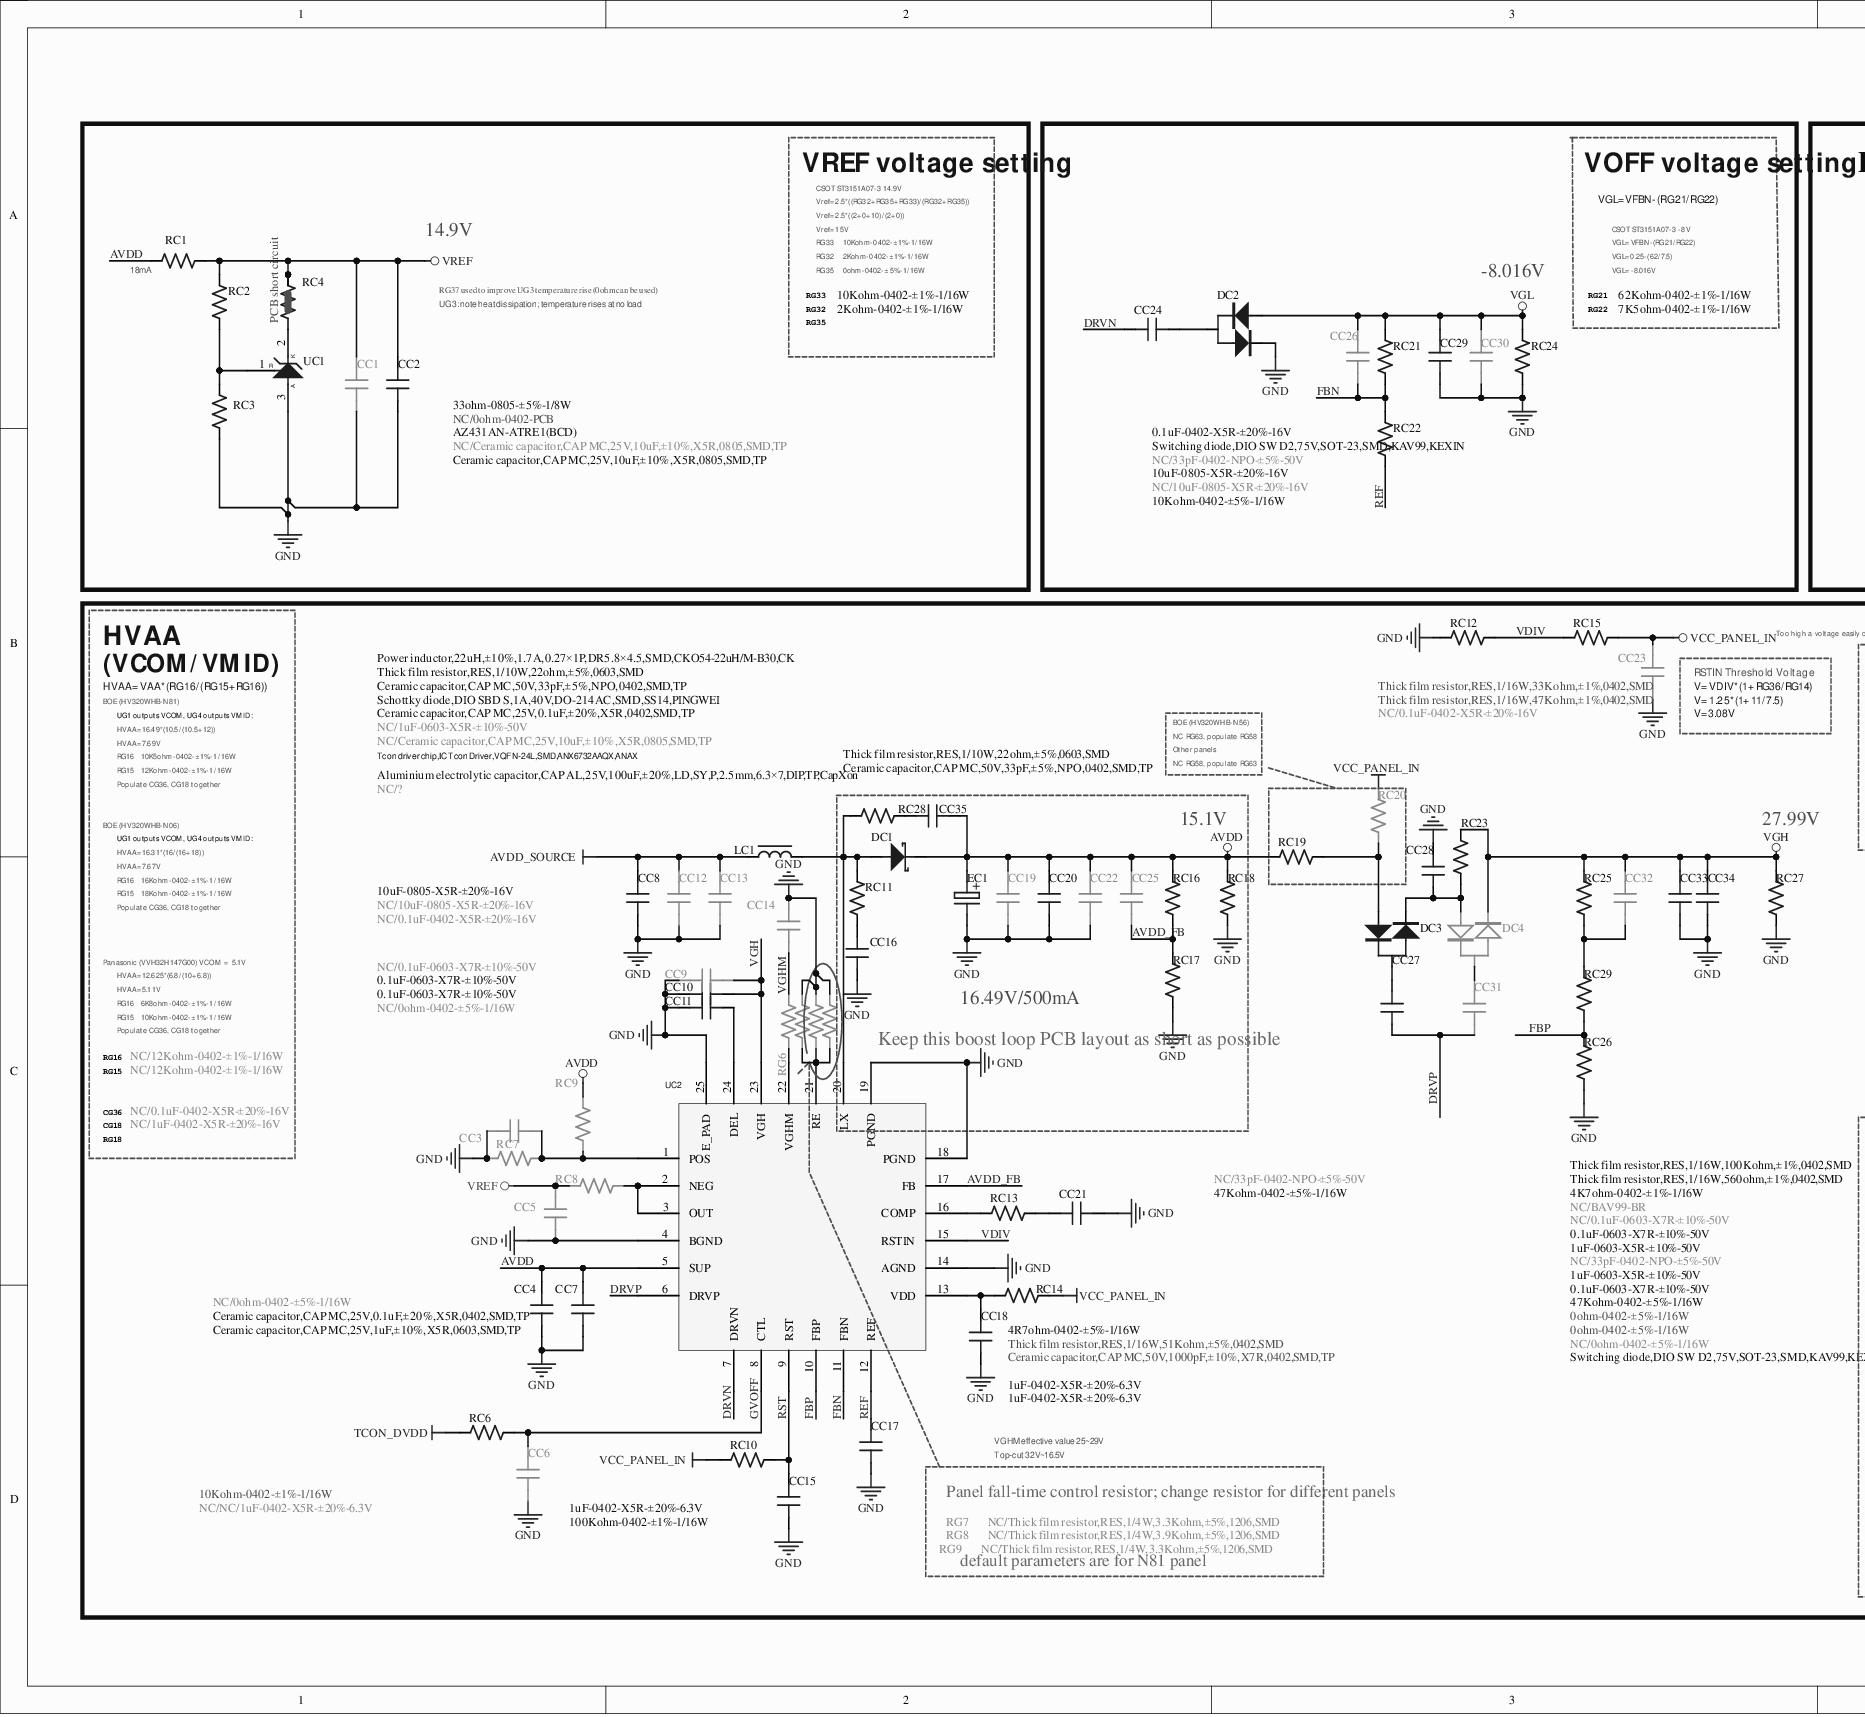
[diagram p0: MISC84395-18.SchDoc, left]
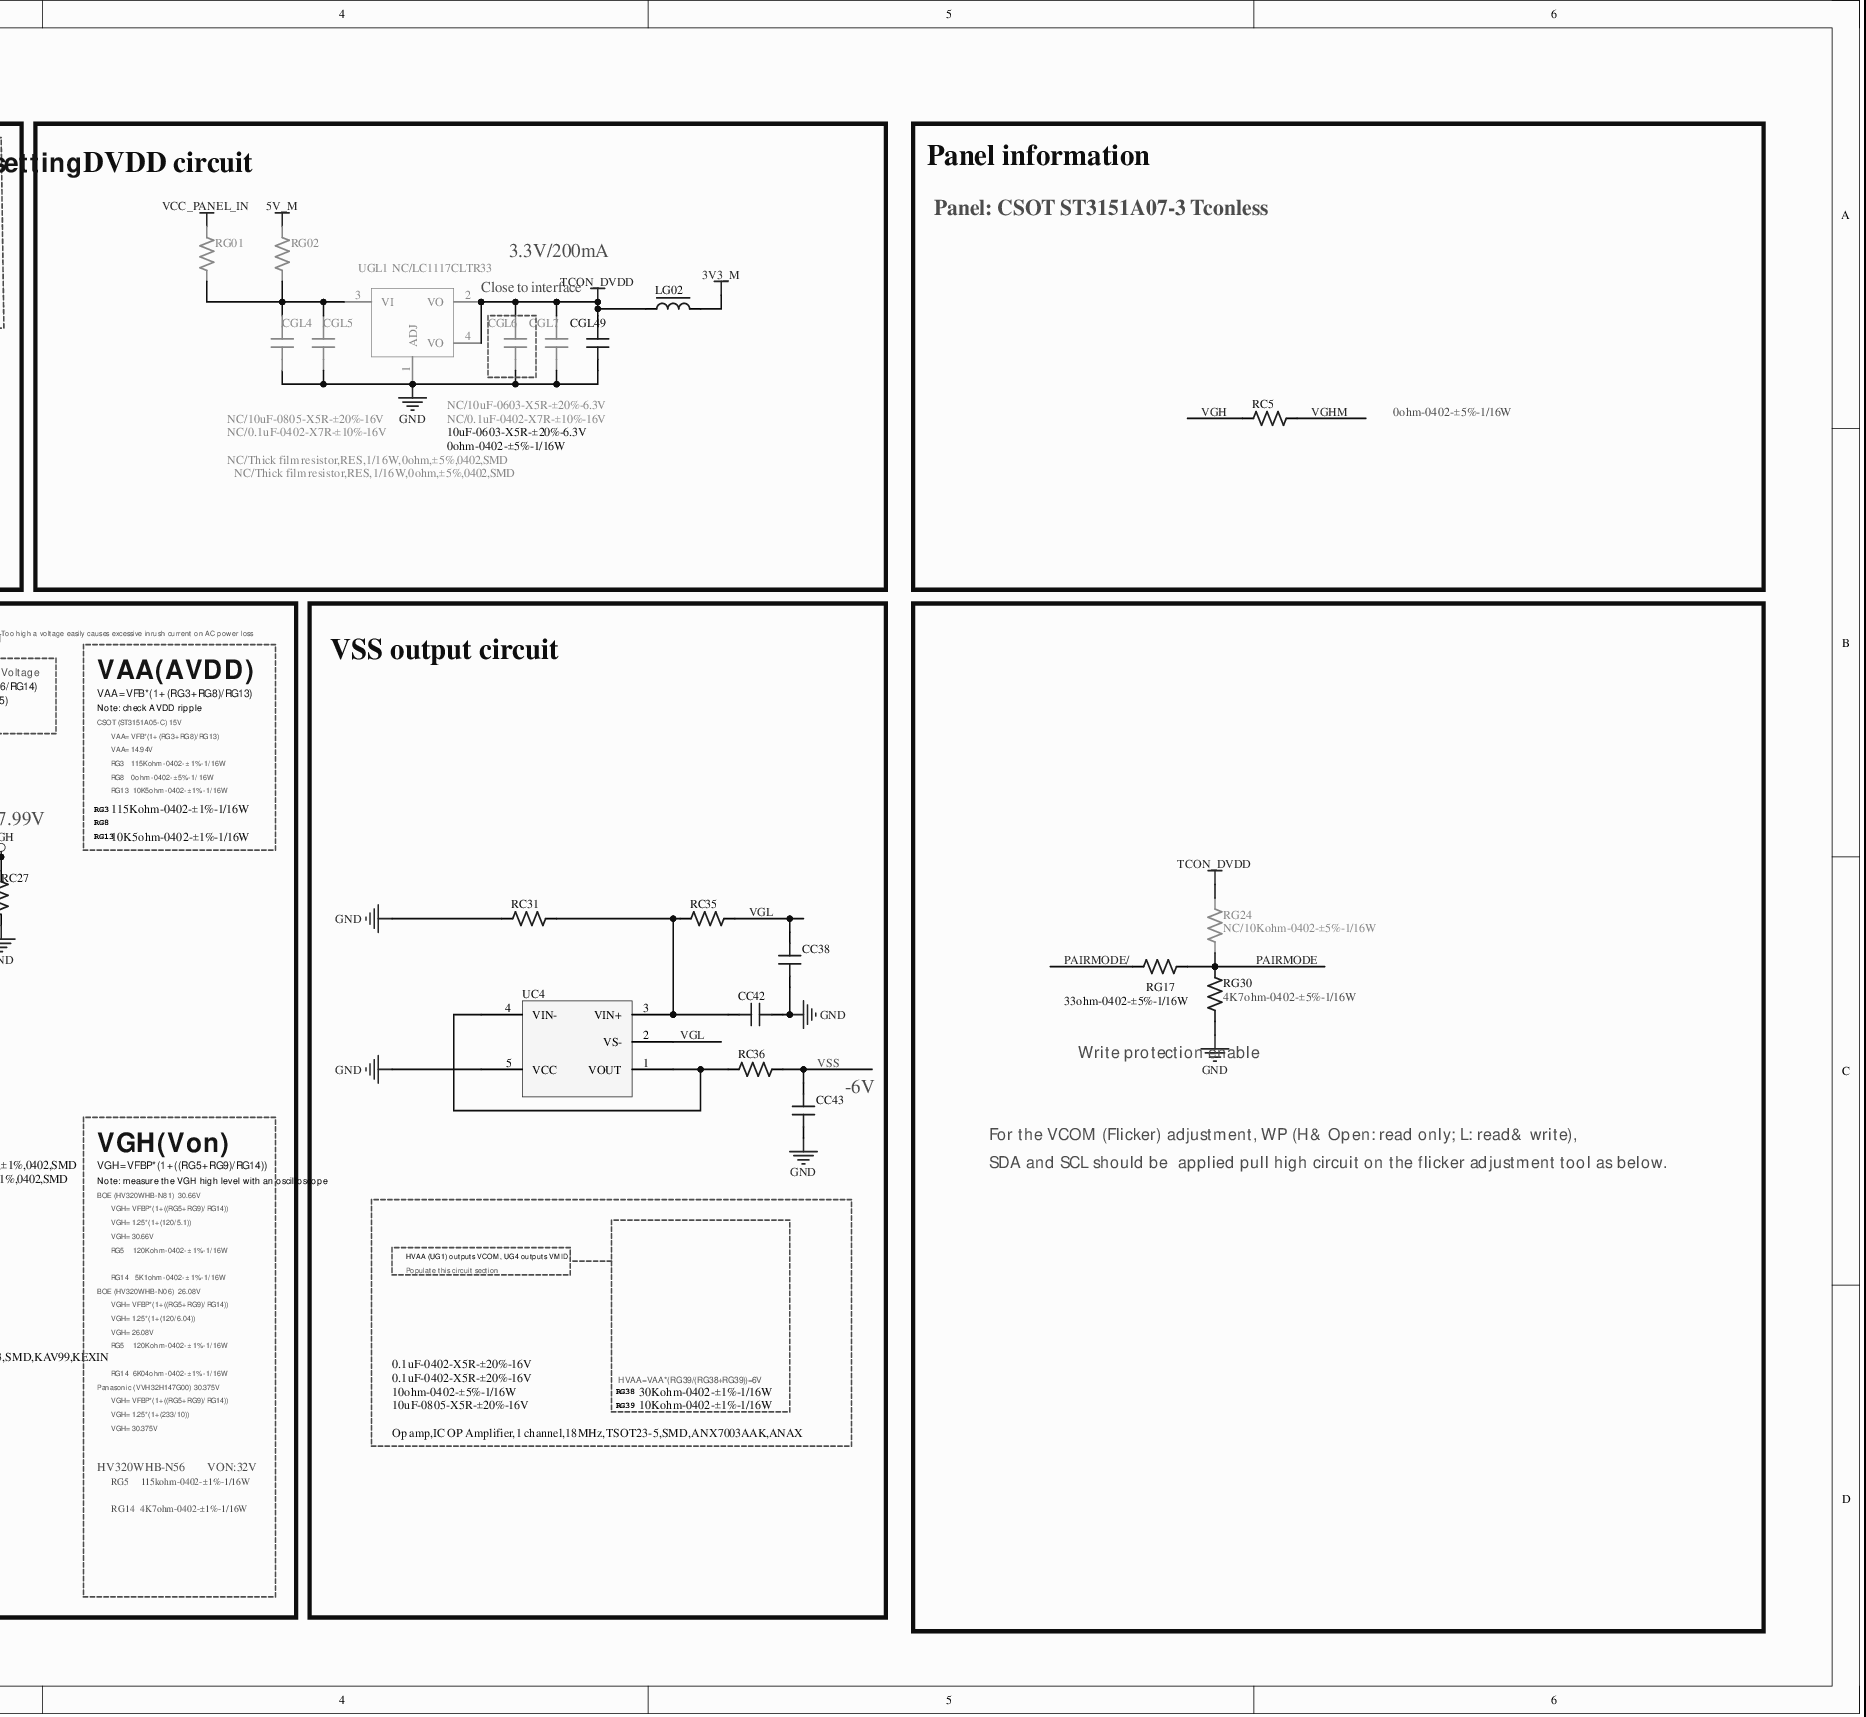
[diagram p1: MISC84395-18.SchDoc, right]
# Altium project MISC84395-37.PrjPCB (part 11 of 13)

## Sheet MISC84395-18.SchDoc
size 673 x 317 mm

### Parts
CC1  NC/Ceramic capacitor,CAP MC,25V,10uF,±10%,X5R,0805,SMD,TP  [C0805]
CC2  Ceramic capacitor,CAP MC,25V,10uF,±10%,X5R,0805,SMD,TP  [C0805]
CC3  NC/0.1uF-0402-X5R-±20%-16V  [C0402]
CC4  Ceramic capacitor,CAP MC,25V,1uF,±10%,X5R,0603,SMD,TP  [C0603]
CC5  NC/1uF-0402-X5R-±20%-16V  [C0402]
CC6  NC/NC/1uF-0402-X5R-±20%-6.3V  [C0402]
CC7  Ceramic capacitor,CAP MC,25V,0.1uF,±20%,X5R,0402,SMD,TP  [C0402]
CC8  10uF-0805-X5R-±20%-16V  [C0805]
CC9  NC/0.1uF-0603-X7R-±10%-50V  [C0603]
CC10  0.1uF-0603-X7R-±10%-50V  [C0603]
CC11  0.1uF-0603-X7R-±10%-50V  [C0603]
CC12  NC/10uF-0805-X5R-±20%-16V  [C0805]
CC13  NC/0.1uF-0402-X5R-±20%-16V  [C0402]
CC14  NC/?  [C0805]
CC15  1uF-0402-X5R-±20%-6.3V  [C0402]
CC16  Ceramic capacitor,CAP MC,50V,33pF,±5%,NPO,0402,SMD,TP  [C0402]
CC17  1uF-0402-X5R-±20%-6.3V  [C0402]
CC18  1uF-0402-X5R-±20%-6.3V  [C0402]
CC19  NC/Ceramic capacitor,CAP MC,25V,10uF,±10%,X5R,0805,SMD,TP  [C0805]
CC20  Ceramic capacitor,CAP MC,25V,0.1uF,±20%,X5R,0402,SMD,TP  [C0402]
CC21  Ceramic capacitor,CAP MC,50V,1000pF,±10%,X7R,0402,SMD,TP  [C0402]
CC22  NC/1uF-0603-X5R-±10%-50V  [C0603]
CC23  NC/0.1uF-0402-X5R-±20%-16V  [C0402]
CC24  0.1uF-0402-X5R-±20%-16V  [C0402]
CC25  NC/33pF-0402-NPO-±5%-50V  [C0402]
CC26  NC/33pF-0402-NPO-±5%-50V  [C0402]
CC27  0.1uF-0603-X7R-±10%-50V  [C0603]
CC28  1uF-0603-X5R-±10%-50V  [C0603]
CC29  10uF-0805-X5R-±20%-16V  [C0805]
CC30  NC/10uF-0805-X5R-±20%-16V  [C0805]
CC31  NC/0.1uF-0603-X7R-±10%-50V  [C0603]
CC32  NC/33pF-0402-NPO-±5%-50V  [C0402]
CC33  1uF-0603-X5R-±10%-50V  [C0603]
CC34  0.1uF-0603-X7R-±10%-50V  [C0603]
CC35  Ceramic capacitor,CAP MC,50V,33pF,±5%,NPO,0402,SMD,TP  [C0402]
CC38  0.1uF-0402-X5R-±20%-16V  [C0402]
CC42  0.1uF-0402-X5R-±20%-16V  [C0402]
CC43  10uF-0805-X5R-±20%-16V  [C0805]
CGL4  NC/10uF-0805-X5R-±20%-16V  [C0805]
CGL5  NC/0.1uF-0402-X7R-±10%-16V  [C0402]
CGL6  NC/10uF-0603-X5R-±20%-6.3V  [C0603]
CGL7  NC/0.1uF-0402-X7R-±10%-16V  [C0402]
CGL49  10uF-0603-X5R-±20%-6.3V  [C0603]
DC1  Schottky diode,DIO SBD S,1A,40V,DO-214AC,SMD,SS14,PINGWEI  [DIODE-S-1]
DC2  Switching diode,DIO SW D2,75V,SOT-23,SMD,KAV99,KEXIN  [SO-23]
DC3  Switching diode,DIO SW D2,75V,SOT-23,SMD,KAV99,KEXIN  [SO-23]
DC4  NC/BAV99-BR  [SO-23]
EC1  Aluminium electrolytic capacitor,CAP AL,25V,100uF,±20%,LD,SY,P,2.5mm,6.3×7,DIP,TP,CapXon  [EC(6.3*11)-V-2.5]
LC1  Power inductor,22uH,±10%,1.7A,0.27×1P,DR5.8×4.5,SMD,CKO54-22uH/M-B30,CK  [L(5.8*4.5)-S]
LG02  0ohm-0402-±5%-1/16W  [L0402]
RC1  33ohm-0805-±5%-1/8W  [R0805]
RC2  10Kohm-0402-±1%-1/16W  [R0402]
RC3  2Kohm-0402-±1%-1/16W  [R0402]
RC4  NC/0ohm-0402-PCB  [R0402SC]
RC5  0ohm-0402-±5%-1/16W  [R0402]
RC6  10Kohm-0402-±1%-1/16W  [R0402]
RC7  NC/12Kohm-0402-±1%-1/16W  [R0402]
RC8  NC/0ohm-0402-±5%-1/16W  [R0402]
RC9  NC/12Kohm-0402-±1%-1/16W  [R0402]
RC10  100Kohm-0402-±1%-1/16W  [R0402]
RC11  Thick film resistor,RES,1/10W,22ohm,±5%,0603,SMD  [R0603]
RC12  Thick film resistor,RES,1/16W,33Kohm,±1%,0402,SMD  [R0402]
RC13  Thick film resistor,RES,1/16W,51Kohm,±5%,0402,SMD  [R0402]
RC14  4R7ohm-0402-±5%-1/16W  [R0402]
RC15  Thick film resistor,RES,1/16W,47Kohm,±1%,0402,SMD  [R0402]
RC16  115Kohm-0402-±1%-1/16W  [R0402]
RC17  10K5ohm-0402-±1%-1/16W  [R0402]
RC18  47Kohm-0402-±5%-1/16W  [R0402]
RC19  0ohm-0402-±5%-1/16W  [R0402]
RC20  NC/0ohm-0402-±5%-1/16W  [R0402]
RC21  62Kohm-0402-±1%-1/16W  [R0402]
RC22  7K5ohm-0402-±1%-1/16W  [R0402]
RC23  0ohm-0402-±5%-1/16W  [R0402]
RC24  10Kohm-0402-±5%-1/16W  [R0402]
RC25  Thick film resistor,RES,1/16W,100Kohm,±1%,0402,SMD  [R0402]
RC26  4K7ohm-0402-±1%-1/16W  [R0402]
RC27  47Kohm-0402-±5%-1/16W  [R0402]
RC28  Thick film resistor,RES,1/10W,22ohm,±5%,0603,SMD  [R0603]
RC29  Thick film resistor,RES,1/16W,560ohm,±1%,0402,SMD  [R0402]
RC31  30Kohm-0402-±1%-1/16W  [R0402]
RC35  10Kohm-0402-±1%-1/16W  [R0402]
RC36  10ohm-0402-±5%-1/16W  [R0402]
RG01  NC/Thick film resistor,RES,1/16W,0ohm,±5%,0402,SMD  [R0402]
RG02  NC/Thick film resistor,RES,1/16W,0ohm,±5%,0402,SMD  [R0402]
RG6  NC/0ohm-0402-±5%-1/16W  [R0402]
RG7  NC/Thick film resistor,RES,1/4W,3.3Kohm,±5%,1206,SMD  [R1206]
RG8  NC/Thick film resistor,RES,1/4W,3.9Kohm,±5%,1206,SMD  [R1206]
RG9  NC/Thick film resistor,RES,1/4W,3.3Kohm,±5%,1206,SMD  [R1206]
RG17  33ohm-0402-±5%-1/16W  [R0402]
RG24  NC/10Kohm-0402-±5%-1/16W  [R0402]
RG30  4K7ohm-0402-±5%-1/16W  [R0402]
UC1  AZ431AN-ATRE1(BCD)  [SO-23-1]
UC2  Tcon driver chip,IC Tcon Driver,VQFN-24L,SMD,ANX6732AAQX,ANAX  [QFN24/0.5-5]
UC4  Op amp,IC OP Amplifier,1 channel,18MHz,TSOT23-5,SMD,ANX7003AAK,ANAX  [SOT-23-5]
UGL1  NC/LC1117CLTR33  [SOT-223]

### Blocks framed on the sheet
VREF voltage setting: CC1 CC2 RC1-RC4 UC1
VOFF voltage setting: CC24 CC26 CC29 CC30 DC2 RC21 RC22 RC24
DVDD circuit: CGL4-CGL7 CGL49 LG02 RG01 RG02 UGL1
Panel information: RC5
VSS output circuit: CC38 CC42 CC43 RC31 RC35 RC36 UC4
Write protection enable: RG17 RG24 RG30

### Nets
3V3_M: LG02.2
5V_M: RG02.2
AVDD: CC4.1 CC7.2 CC19.1 CC20.2 CC22.1 CC25.2 CC35.1 DC1.K EC1.1 RC1.1 RC9.2 RC16.2 RC18.2 RC19.2 UC2.5(SUP)
AVDD_SOURCE: CC8.1 CC12.1 CC13.2 LC1.1
GND: CC1.1 CC2.1 CC3.2 CC4.2 CC5.2 CC6.1 CC7.1 CC8.2 CC9.2 CC10.2 CC11.2 CC12.2 CC13.1 CC14.1 CC15.1 CC16.1 CC17.1 CC18.1 CC19.2 CC20.1 CC21.2 CC22.2 CC23.1 CC28.2 CC29.2 CC30.2 CC33.1 CC34.1 CC38.2 CC42.2 CC43.1 CGL4.1 CGL5.2 CGL6.2 CGL7.2 CGL49.2 DC2.3 EC1.2 RC3.1 RC7.2 RC12.1 RC17.1 RC18.1 RC24.1 RC26.1 RC27.1 RC31.1 RG7.2 RG8.2 RG9.2 RG30.2 UC1.3(A) UC2.4(BGND) UC2.14(AGND) UC2.18(PGND) UC2.19(PGND) UC2.25(E_PAD) UC4.5(VCC) UGL1.1(ADJ)
TCON_DVDD: CGL6.1 CGL7.1 CGL49.1 LG02.1 RC6.2 RG24.1 UGL1.2(VO) UGL1.4(VO)
VCC_PANEL_IN: CC23.2 RC10.2 RC14.2 RC15.2 RC20.1 RG01.2
VGH: CC9.1 CC10.1 CC32.2 CC33.2 CC34.2 DC4.3 RC5.2 RC23.2 RC25.2 RC27.2 UC2.23(VGH)
VGL: CC26.2 CC29.1 CC30.1 CC38.1 DC2.1 RC21.2 RC24.2 RC35.2 UC4.2(VS-)
VREF: CC1.2 CC2.2 CC5.1 RC1.2 RC2.2 RC4.2 RC4.3 RC8.1
AVDD_FB: CC25.1 RC16.1 RC17.2 UC2.17(FB)
DRVN: CC24.1 UC2.7(DRVN)
DRVP: CC27.2 CC31.2 UC2.6(DRVP)
FBN: CC26.1 RC21.1 RC22.2 UC2.11(FBN)
FBP: RC26.2 RC29.1 UC2.10(FBP)
GVOFF: CC6.2 RC6.1 UC2.8(CTL)
PAIRMODE: RG17.2 RG24.2 RG30.1
PAIRMODE/: RG17.1
REF: CC17.2 RC22.1 UC2.12(REF)
RST: CC15.2 RC10.1 UC2.9(RST)
VDIV: RC12.2 RC15.1 UC2.15(RSTIN)
VGHM: CC14.2 RC5.1 RG6.2
VSS: CC43.2 RC36.2
NetCC3_1: CC3.1 RC7.1 RC9.1 UC2.1(POS)
NetCC11_1: CC11.1 UC2.24(DEL)
NetCC16_2: CC16.2 RC11.1
NetCC18_2: CC18.2 RC14.1 UC2.13(VDD)
NetCC21_1: CC21.1 RC13.2
NetCC24_2: CC24.2 DC2.2
NetCC27_1: CC27.1 DC3.2
NetCC28_1: CC28.1 DC3.3 DC4.1 RC23.1
NetCC31_1: CC31.1 DC4.2
NetCC32_1: CC32.1 RC25.1 RC29.2
NetCC35_2: CC35.2 RC28.1
NetCC42_1: CC42.1 RC31.2 RC35.1 UC4.3(VIN+)
NetCGL4_2: CGL4.2 CGL5.1 RG01.1 RG02.1 UGL1.3(VI)
NetDC1_A: DC1.A LC1.2 RC11.2 RC28.2 UC2.20(LX)
NetDC3_1: DC3.1 RC19.1 RC20.2
NetRC2_1: RC2.1 RC3.2 UC1.1(R)
NetRC4_1: RC4.1 UC1.2(K)
NetRC8_2: RC8.2 UC2.2(NEG) UC2.3(OUT)
NetRC13_1: RC13.1 UC2.16(COMP)
NetRC36_1: RC36.1 UC4.1(VOUT) UC4.4(VIN-)
NetRG6_1: RG6.1 UC2.22(VGHM)
NetRG7_1: RG7.1 RG8.1 RG9.1 UC2.21(RE)

### Notes on the sheet
- 14.9V
- Vref=2.5*((RG32+RG35+RG33)/(RG32+RG35))
- Vref=2.5*((2+0+10)/(2+0))
- Vref=15V
- CSOT ST3151A07-3 14.9V
- VGL=VFBN-(RG21/RG22)
- CSOT ST3151A07-3 -8V
- Panel: CSOT ST3151A07-3 Tconless
- (near RC1) 18mA
- RG37 used to improve UG3 temperature rise (0ohm can be used)
- RG33
- RG33    10Kohm-0402-±1%-1/16W
- RG32    2Kohm-0402-±1%-1/16W
- RG35    0ohm-0402-±5%-1/16W
- -8.016V
- RG21
- VGL=0.25-(62/7.5)
- VGL=-8.016V
- Close to interface
- 3.3V/200mA
- UG3: note heat dissipation; temperature rises at no load
- RG32
- RG35
- RG22
- HVAA
- Too high a voltage easily causes excessive inrush current on AC power loss
- BOE (HV320WHB-N81)
- HVAA=VAA*(RG16/(RG15+RG16))
- (VCOM/VMID)
- (near CC23) V=VDIV*(1+RG36/RG14)
- (near CC23) V=1.25*(1+11/7.5)
- (near CC23) RSTIN Threshold Voltage
- VAA(AVDD)
- VAA=VFB*(1+(RG3+RG8)/RG13)
- Note: check AVDD ripple
- RG15   12Kohm-0402-±1%-1/16W
- RG16   10K5ohm-0402-±1%-1/16W
- HVAA=16.49*(10.5/(10.5+12))
- HVAA=7.69V
- Populate CG36, CG18 together
- UG1 outputs VCOM, UG4 outputs VMID:
- NC RG58, populate RG63
- BOE (HV320WHB-N56)
- NC RG63, populate RG58
- Other panels
- (near CC23) V=3.08V
- CSOT (ST3151A05-C) 15V
- VAA=14.94V
- RG3   115Kohm-0402-±1%-1/16W
- RG8   0ohm-0402-±5%-1/16W
- BOE (HV320WHB-N06)
- 15.1V
- 27.99V
- RG3
- RG8
- RG13
- RG13  10K5ohm-0402-±1%-1/16W
- RG16   16Kohm-0402-±1%-1/16W
- RG15   18Kohm-0402-±1%-1/16W
- HVAA=16.31*(16/(16+18))
- HVAA=7.67V
- Panasonic (VVH32H147G00) VCOM = 5.1V
- HVAA=12.625*(6.8/(10+6.8))
- RG16
- RG16   6K8ohm-0402-±1%-1/16W
- RG15   10Kohm-0402-±1%-1/16W
- HVAA=5.11V
- (near CC27) Keep this boost loop PCB layout as short as possible
- 16.49V/500mA
- RG15
- CG36
- (near CC43) -6V
- RG18
- CG18
- VGH(Von)
- BOE (HV320WHB-N81)  30.66V
- Note: measure the VGH high level with an oscilloscope
- VGH=VFBP*(1+((RG5+RG9)/RG14))
- For the VCOM (Flicker) adjustment, WP (H& Open: read only; L: read& write),
- SDA and SCL should be  applied pull high circuit on the flicker adjustment tool as below.
- VGH=1.25*(1+(120/5.1))
- VGH=30.66V
- RG5    120Kohm-0402-±1%-1/16W
- HVAA (UG1) outputs VCOM, UG4 outputs VMID:
- BOE (HV320WHB-N06)  26.08V
- VGH=1.25*(1+(120/6.04))
- VGH=26.08V
- RG14   5K1ohm-0402-±1%-1/16W
- Populate this circuit section
- Panasonic (VVH32H147G00) 30.375V
- RG14  6K04ohm-0402-±1%-1/16W
- RG38
- HVAA=VAA*(RG39/(RG38+RG39))=6V
- VGHM effective value 25~29V
- Top-cut 32V~16.5V
- HV320WHB-N56
- VGH=1.25*(1+(233/10))
- VGH=30.375V
- VON:32V
- RG39
- Panel fall-time control resistor; change resistor for different panels
- RG5     115kohm-0402-±1%-1/16W
- RG14   4K7ohm-0402-±1%-1/16W
- default parameters are for N81 panel

### Library data of the parts
CC1 CC2 CC14 CC19 = 22uF-0805-X5R-±20%-6.3V-D
CC3 CC13 CC20 CC38 = 0.1uF-0402-Y5V-+80%-20%-16V-D
CC4 CC22 CC28 CC33 = 1uF-0603-X5R-±10%-50V-D
CC5 = 1uF-0402-X5R-±20%-16V-D
CC6 CC7 CC15 CC17 CC18 = 1uF-0402-X5R-±20%-6.3V-D
CC8 CC12 CC29 CC30 CC43 CGL4 = 10uF-0805-X5R-±20%-16V-D
CC9-CC11 CC27 CC31 CC34 = 0.1uF-0603-X7R-±10%-50V-D: CAP
CC16 CC35 = 68pF-0402-NPO-±5%-50V-D
CC21 = 1500pF-0402-X7R-±10%-50V-D: CAP
CC23 CC24 CC42 = 0.1uF-0402-X5R-±20%-16V-D
CC25 CC26 CC32 = 33pF-0402-NPO-±5%-50V-D
CGL5 CGL7 = 0.1uF-0402-X7R-±10%-16V-D
CGL6 CGL49 = 10uF-0603-X5R-±20%-6.3V-D
DC1 = SK34A-SMA-F-D
DC2-DC4 = BAT54S-D
EC1 = 100uF-35V-±20%-6.3×11-105℃-KF-编带-F=2.5(CapXon)-DHAI: Electrolytic
LC1 = SCD54TL-6R8M-D
LG02 = FCM1005KF-121T06(120ohm-500mA)-D
RC1 = 10ohm-0805-±5%-1/8W-D
RC2 = 12Kohm-0402-±1%-1/16W-D
RC3 = 1K2ohm-0402-±1%-1/16W-D
RC4 = 0ohm-0402-PCB-D
RC5 RC8 RC19 RC20 RC23 RG6 = 0ohm-0402-±5%-1/16W-D
RC6 RC10 = 100Kohm-0402-±5%-1/16W-D
RC7 RC9 = 18Kohm-0402-±1%-1/16W-D
RC11 RC28 = 10ohm-0603-±5%-1/10W-D
RC12 = 56Kohm-0402-±1%-1/16W-D
RC13 RC18 RC27 = 47Kohm-0402-±5%-1/16W-D
RC14 = 4R7ohm-0402-±5%-1/16W-D
RC15 = 121Kohm-0402-±1%-1/16W-D
RC16 = 470Kohm-0402-±1%-1/16W-D
RC17 = 39Kohm-0402-±1%-1/16W-D: RES
RC21 = 62Kohm-0402-±1%-1/16W-D
RC22 = 7K5ohm-0402-±1%-1/16W-D
RC24 RG24 RG30 = 10Kohm-0402-±5%-1/16W-D
RC25 = 100Kohm-0402-±1%-1/16W-D
RC26 RC29 = 6K2ohm-0402-±1%-1/16W-D
RC31 = 16Kohm-0402-±1%-1/16W-D
RC35 = 9K1ohm-0402-±1%-1/16W-D
RC36 = 10ohm-0402-±5%-1/16W-D
RG01 RG02 = 004.002.0000558-D: Thick film resistor,RES,1/16W,0ohm,±5%,0402,SMD-D
RG7 RG9 = 1Kohm-1206-±5%-1/4W-D
RG8 = 470ohm-1206-±5%-1/4W-D: RES
RG17 = 33ohm-0402-±5%-1/16W-D
UC1 = TL431G-AE2-R(UTC)-D
UC2 = G5517-D
UC4 = 运算放大器,IC OP Amplifier,1 channel,18MHz,TSOT23-5,SMD,ANX7003AAK,ANAX
UGL1 = LC1117CLTR33-D